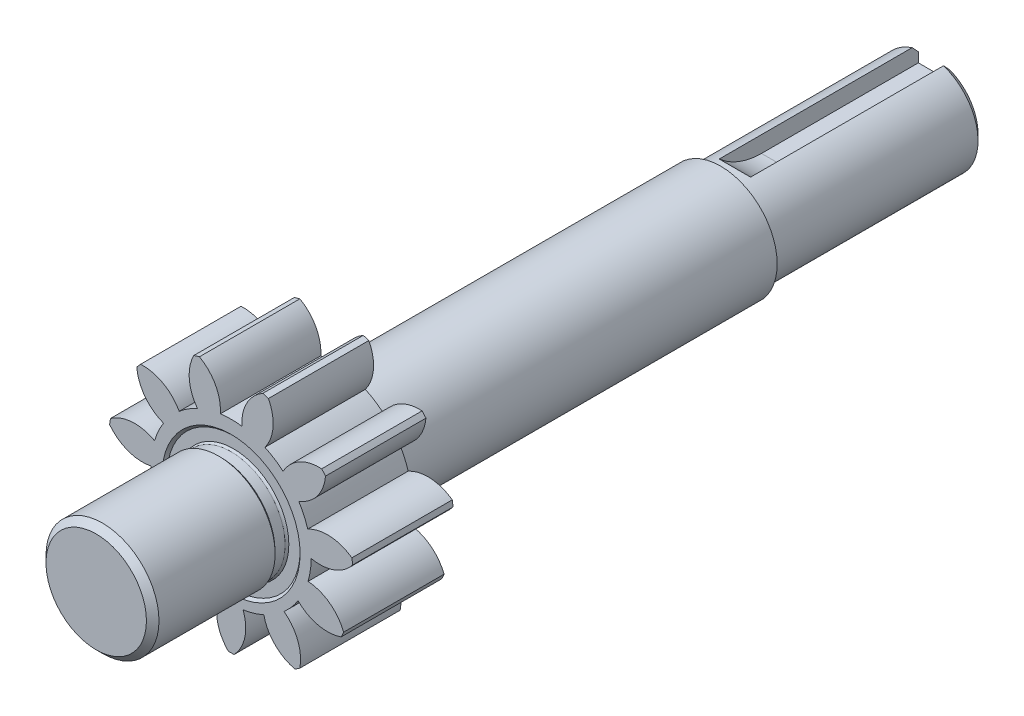
SolidWorks part; units mm, degrees
ref_plane "前视基准面" through (0, 0, 0) normal (0, 0, 1) x (1, 0, 0)
ref_plane "上视基准面" through (0, 0, 0) normal (0, 1, 0) x (1, 0, 0)
ref_plane "右视基准面" through (0, 0, 0) normal (1, 0, 0) x (0, 0, -1)
sketch "草图1" plane through (0, 0, 0) normal (0, 0, 1) x (1, 0, 0)
  arc A0 (-17.5397, -8.1889) -> (-10.6725, -6.6417) centre (-15.3333, -1.9687) ccw
  arc A1 (-10.6725, -6.6417) -> (-8.4217, -9.2393) centre (0, 0.3321) ccw
  arc A2 (-8.4217, -9.2393) -> (-10.9305, -15.8164) centre (-4.4595, -14.5176) ccw
  arc A3 (-10.9305, -15.8164) -> (-10.1485, -16.3189) centre (0, 0.3321) ccw
  arc A4 (-10.1485, -16.3189) -> (-5.2079, -11.3046) centre (-11.6553, -9.8932) ccw
  arc A5 (-5.2079, -11.3046) -> (-1.9101, -12.273) centre (0, 0.3321) ccw
  arc A6 (-1.9101, -12.273) -> (-0.4648, -19.1623) centre (4.2768, -14.5713) ccw
  arc A7 (-0.4648, -19.1623) -> (0.4648, -19.1623) centre (0, 0.3321) ccw
  arc A8 (0.4648, -19.1623) -> (1.9101, -12.273) centre (-4.2768, -14.5713) ccw
  arc A9 (1.9101, -12.273) -> (5.2079, -11.3046) centre (0, 0.3321) ccw
  arc A10 (5.2079, -11.3046) -> (10.1485, -16.3189) centre (11.6553, -9.8932) ccw
  arc A11 (10.1485, -16.3189) -> (10.9305, -15.8164) centre (0, 0.3321) ccw
  arc A12 (10.9305, -15.8164) -> (8.4217, -9.2393) centre (4.4595, -14.5176) ccw
  arc A13 (8.4217, -9.2393) -> (10.6725, -6.6417) centre (0, 0.3321) ccw
  arc A14 (10.6725, -6.6417) -> (17.5397, -8.1889) centre (15.3333, -1.9687) ccw
  arc A15 (17.5397, -8.1889) -> (17.9259, -7.3434) centre (0, 0.3321) ccw
  arc A16 (17.9259, -7.3434) -> (12.2595, -3.1667) centre (11.78, -9.7493) ccw
  arc A17 (12.2595, -3.1667) -> (12.7486, 0.2354) centre (0, 0.3321) ccw
  arc A18 (12.7486, 0.2354) -> (19.3622, 2.6465) centre (14.1431, 6.6864) ccw
  arc A19 (19.3622, 2.6465) -> (19.2299, 3.5665) centre (0, 0.3321) ccw
  arc A20 (19.2299, 3.5665) -> (12.205, 4.0167) centre (15.3604, -1.7802) ccw
  arc A21 (12.205, 4.0167) -> (10.7771, 7.1432) centre (0, 0.3321) ccw
  arc A22 (10.7771, 7.1432) -> (15.0373, 12.7471) centre (8.4625, 13.324) ccw
  arc A23 (15.0373, 12.7471) -> (14.4286, 13.4495) centre (0, 0.3321) ccw
  arc A24 (14.4286, 13.4495) -> (8.2754, 10.0303) centre (14.064, 6.8596) ccw
  arc A25 (8.2754, 10.0303) -> (5.384, 11.8885) centre (0, 0.3321) ccw
  arc A26 (5.384, 11.8885) -> (5.9382, 18.906) centre (0.0952, 15.8368) ccw
  arc A27 (5.9382, 18.906) -> (5.0463, 19.1679) centre (0, 0.3321) ccw
  arc A28 (5.0463, 19.1679) -> (1.7185, 12.9648) centre (8.3023, 13.4269) ccw
  arc A29 (1.7185, 12.9648) -> (-1.7185, 12.9648) centre (0, 0.3321) ccw
  arc A30 (-1.7185, 12.9648) -> (-5.0463, 19.1679) centre (-8.3023, 13.4269) ccw
  arc A31 (-5.0463, 19.1679) -> (-5.9382, 18.906) centre (0, 0.3321) ccw
  arc A32 (-5.9382, 18.906) -> (-5.384, 11.8885) centre (-0.0952, 15.8368) ccw
  arc A33 (-5.384, 11.8885) -> (-8.2754, 10.0303) centre (0, 0.3321) ccw
  arc A34 (-8.2754, 10.0303) -> (-14.4286, 13.4495) centre (-14.064, 6.8596) ccw
  arc A35 (-14.4286, 13.4495) -> (-15.0373, 12.7471) centre (0, 0.3321) ccw
  arc A36 (-15.0373, 12.7471) -> (-10.7771, 7.1432) centre (-8.4625, 13.324) ccw
  arc A37 (-10.7771, 7.1432) -> (-12.205, 4.0167) centre (0, 0.3321) ccw
  arc A38 (-12.205, 4.0167) -> (-19.2299, 3.5665) centre (-15.3604, -1.7802) ccw
  arc A39 (-19.2299, 3.5665) -> (-19.3622, 2.6465) centre (0, 0.3321) ccw
  arc A40 (-19.3622, 2.6465) -> (-12.7486, 0.2354) centre (-14.1431, 6.6864) ccw
  arc A41 (-12.7486, 0.2354) -> (-12.2595, -3.1667) centre (0, 0.3321) ccw
  arc A42 (-12.2595, -3.1667) -> (-17.9259, -7.3434) centre (-11.78, -9.7493) ccw
  arc A43 (-17.9259, -7.3434) -> (-17.5397, -8.1889) centre (0, 0.3321) ccw
extrude "凸台-拉伸1" add sketch "草图1" along normal blind 16
sketch "草图2" plane through (0, 0, 16) normal (0, 0, 1) x (1, 0, 0)
  circle A0 centre (0, 0) radius 9
  dimension "D1" = 18
extrude "凸台-拉伸2" add sketch "草图2" along normal blind 21.5
sketch "草图3" plane through (0, 0, 0) normal (0, 0, -1) x (-1, 0, 0)
  circle A0 centre (0, 0) radius 9
  dimension "D1" = 18
extrude "凸台-拉伸3" add sketch "草图3" along normal blind 62
sketch "草图4" plane through (0, 0, -62) normal (0, 0, -1) x (-1, 0, 0)
  circle A0 centre (0, 0) radius 8
  dimension "D1" = 16
extrude "凸台-拉伸4" add sketch "草图4" along normal blind 34
sketch "草图5" plane through (0, 0, 0) normal (1, 0, 0) x (0, 0, -1)
  line L0 (-16, 10.9894) -> (-15.6, 10.5894)
  line L1 (-16, 11.8885) -> (-16, 10.0303) construction
  line L2 (-15.6, 10.5894) -> (-15.6, 8.7927)
  line L3 (-18, 8.9894) -> (-17.6, 8.5894)
  line L4 (-17.6, 8.5894) -> (-16, 8.5894)
  line L5 (-16, 9) -> (-16, -9) construction
  line L6 (-16, 10.9894) -> (-18, 10.9894)
  line L7 (-18, 10.9894) -> (-18, 8.9894)
  line L8 (-16, 12.7471) -> (-16, 7.1432) construction
  arc A0 (-15.6, 8.7927) -> (-16, 8.5894) centre (-16.1479, 9.3756) cw
  dimension "D4" = 0.4
  dimension "D8" = 0.8
  dimension "D1" = 135
  dimension "D2" = 45
  dimension "D3" = 2
  dimension "D5" = 2
  dimension "D6" = 2
  dimension "D7" = 0.4
revolve "切除-旋转1" cut sketch "草图5" angle 360 about axis through (0, 0, 37.5) along (0, 0, -1)
ref_plane "基准面1" through (0, 0, 8) normal (0, 0, 1) x (1, 0, 0)
mirror "镜向1" about plane through (0, 0, 8) normal (0, 0, 1) of "切除-旋转1"
sketch "草图6" plane through (0, 0, 0) normal (1, 0, 0) x (0, 0, -1)
  line L0 (96, 12.9401) -> (96, 5)
  line L1 (96, 5) -> (71, 5)
  line L2 (71, 14.4848) -> (71, 5) construction
  line L3 (61.1511, 20.2416) -> (96, 20.2416)
  line L4 (96, 20.2416) -> (96, 12.9401)
  line L5 (96, -8) -> (96, 8) construction
  line L6 (96, 8) -> (62, 8) construction
  line L7 (61.1511, 13.2681) -> (61.1511, 20.2416)
  arc A0 (71, 5) -> (61.1511, 13.2681) centre (71, 15) cw
  dimension "D1" = 25
  dimension "D2" = 3
extrude "切除-拉伸1" cut sketch "草图6" against normal mid plane 5
chamfer "倒角1" distance 1 angle 45 2 edges at (9, 0, 37.5) (0, -8, -96)
